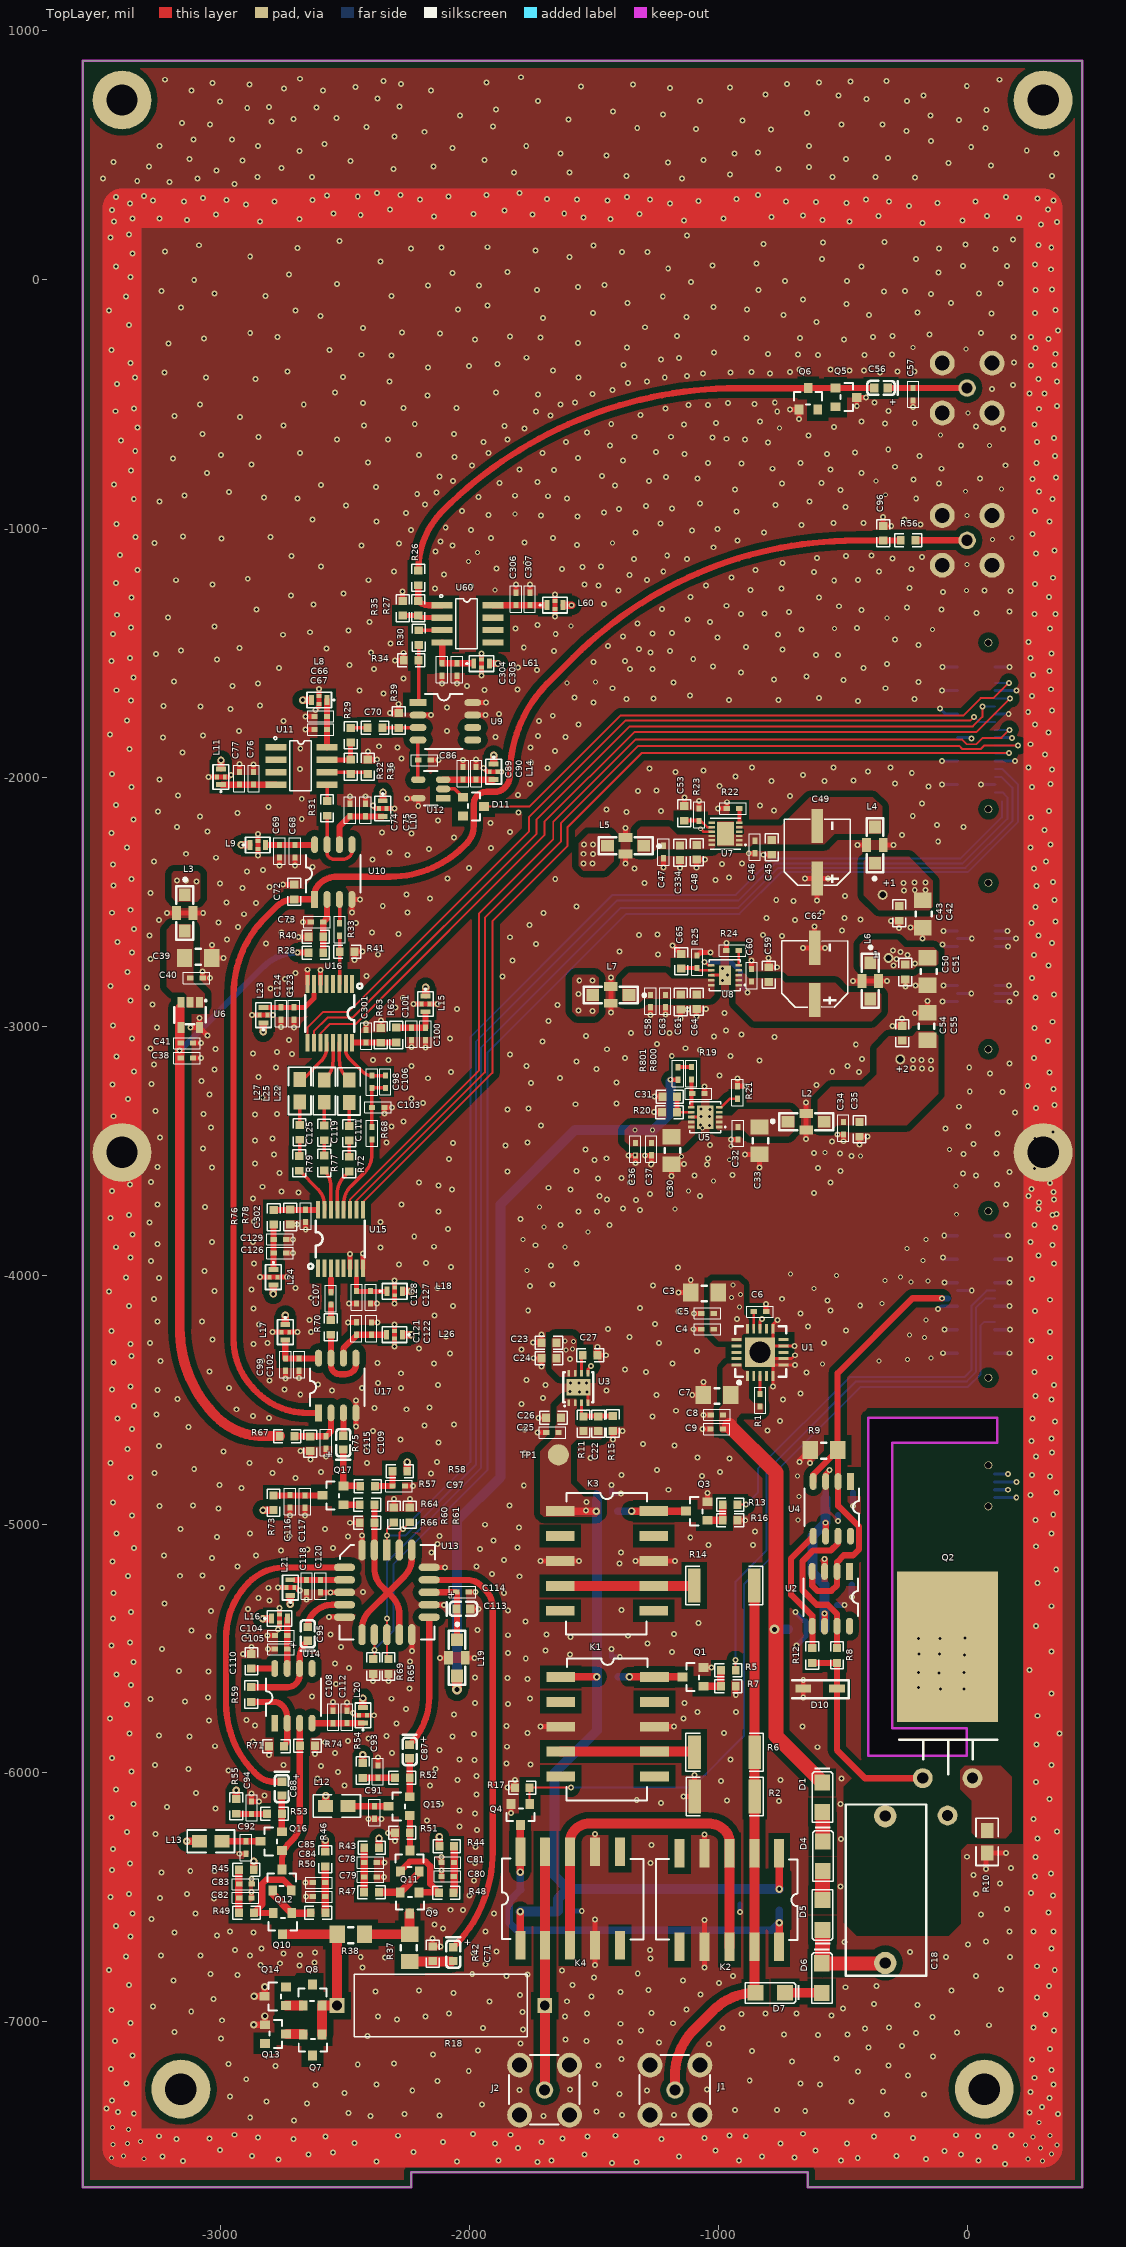
[diagram p0: TopLayer view]
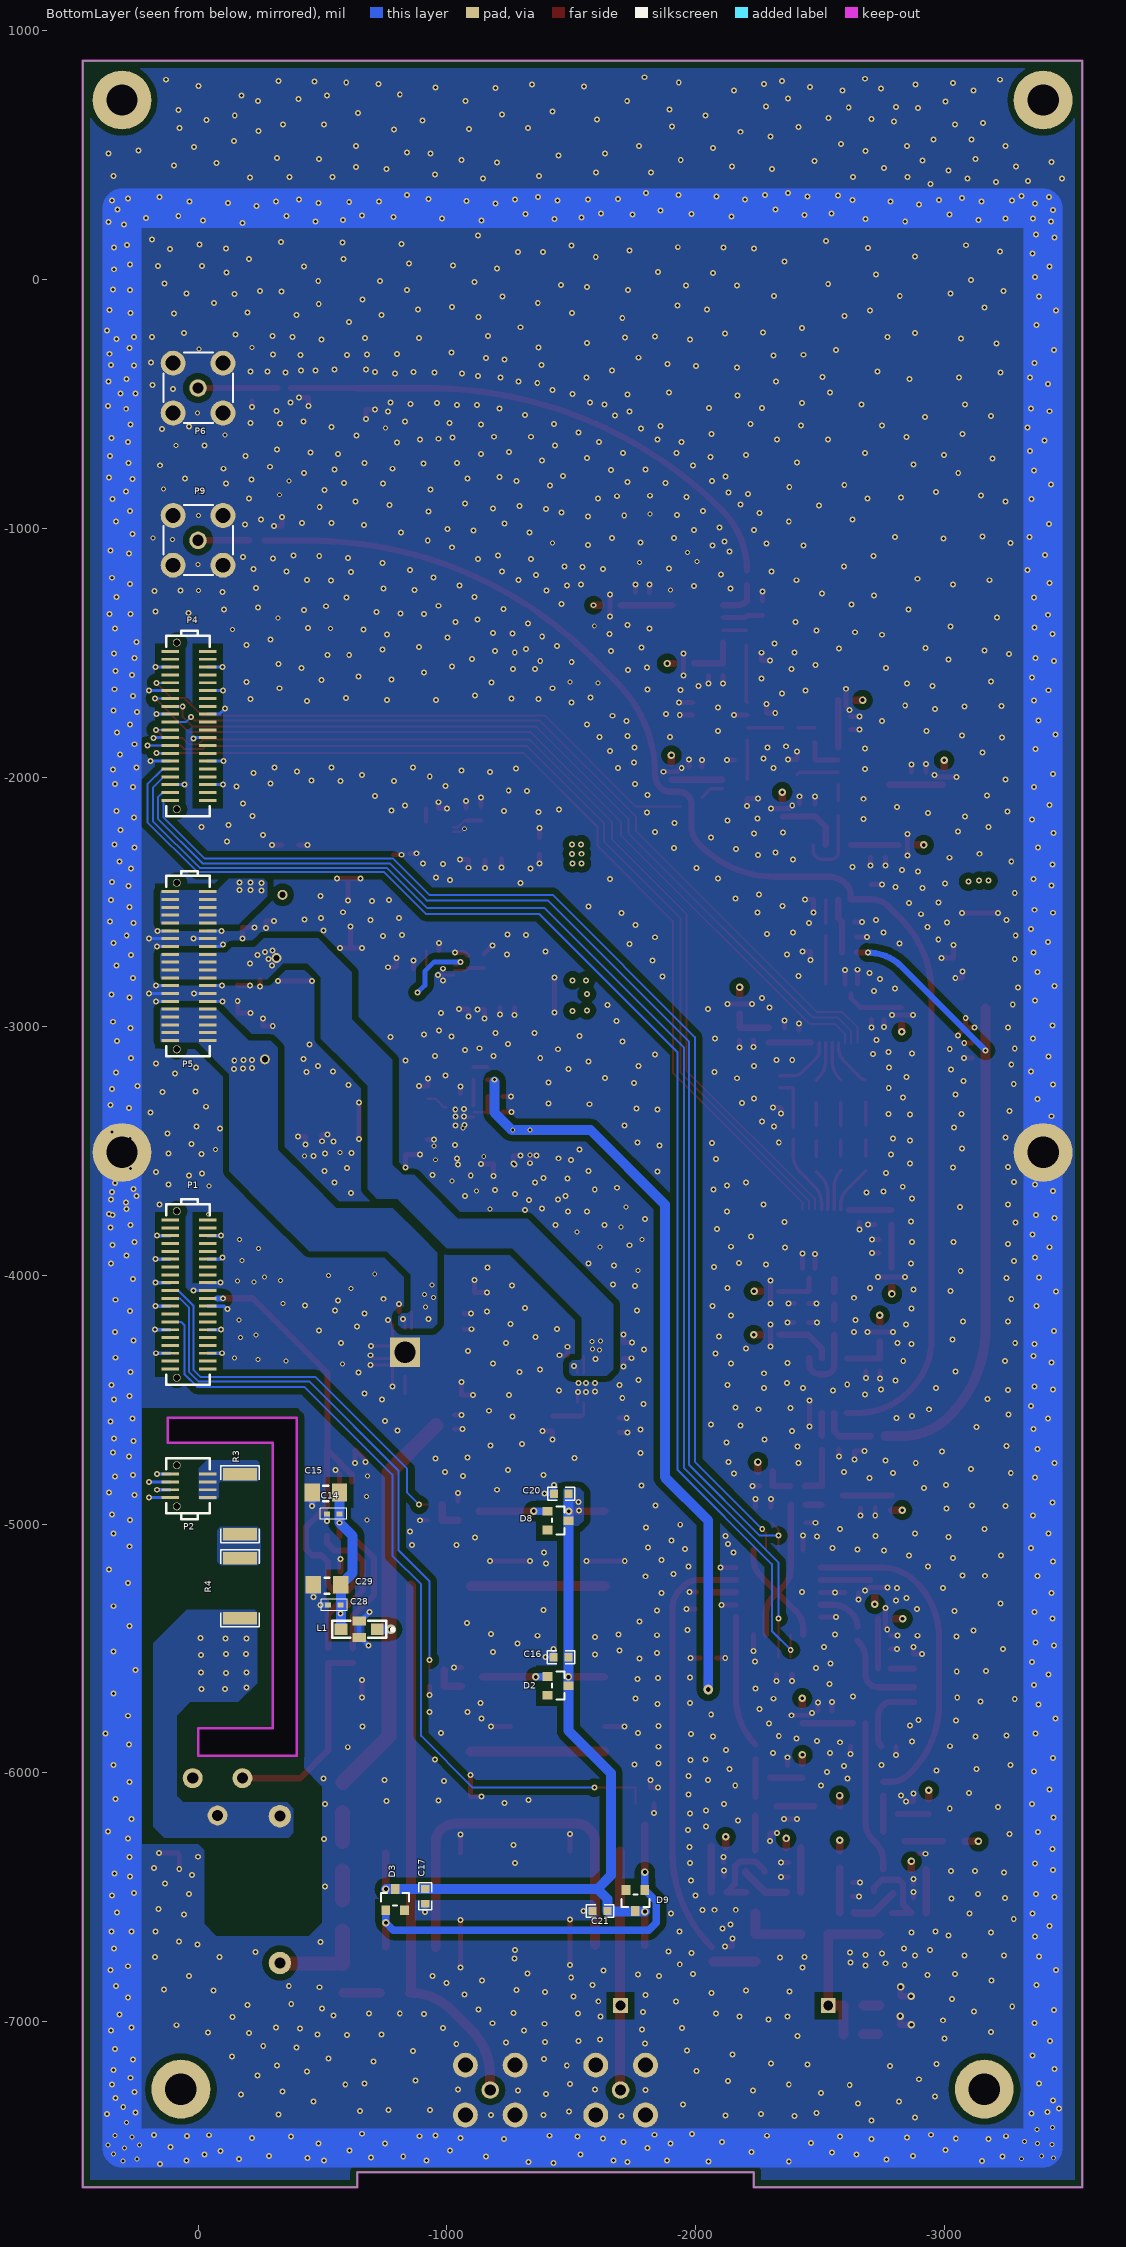
[diagram p1: BottomLayer view, seen from below]
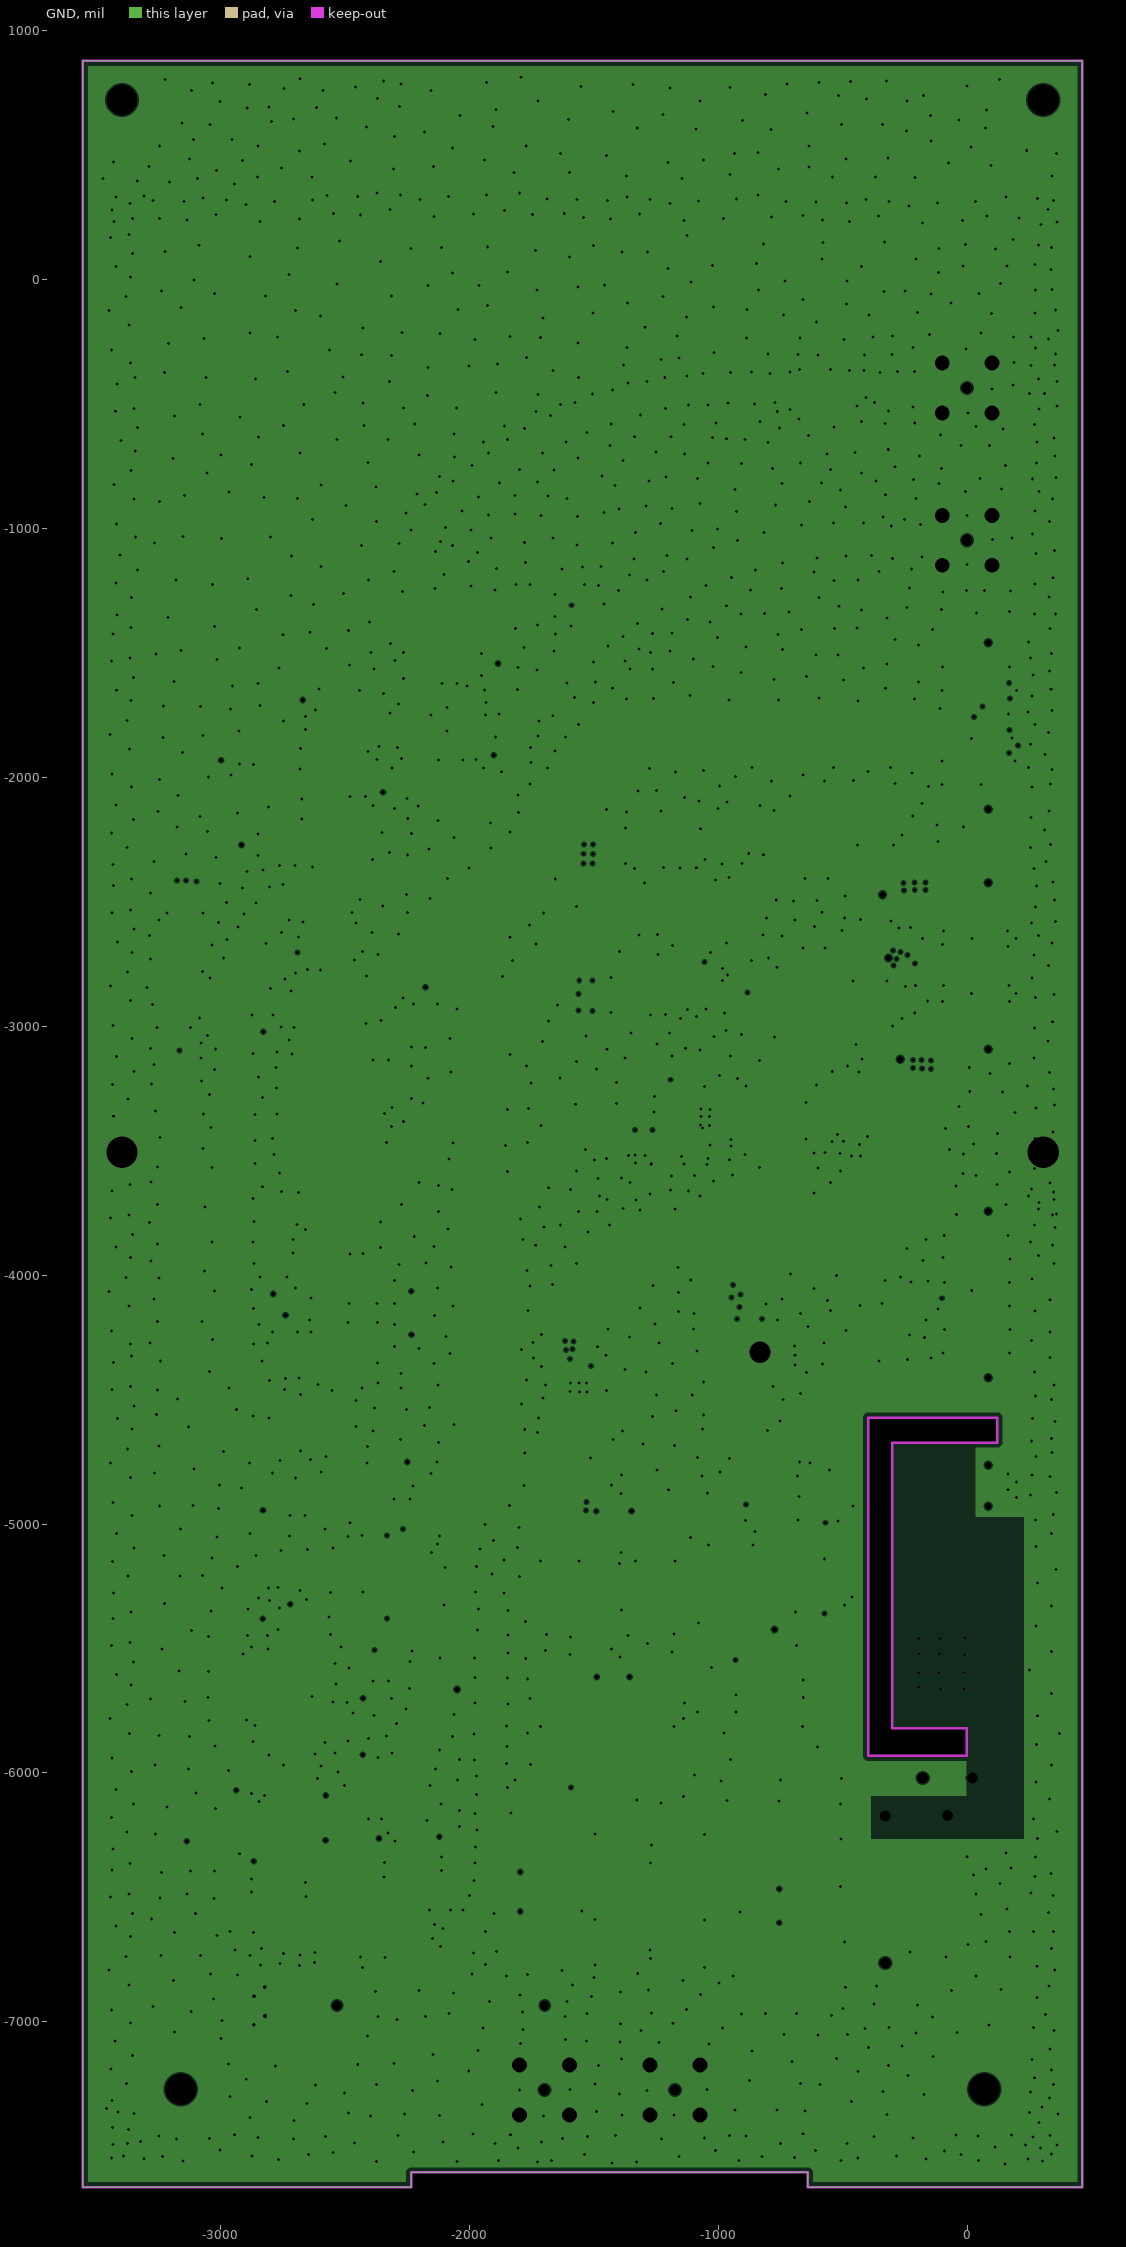
[diagram p2: GND, clearances drawn from the general rule]
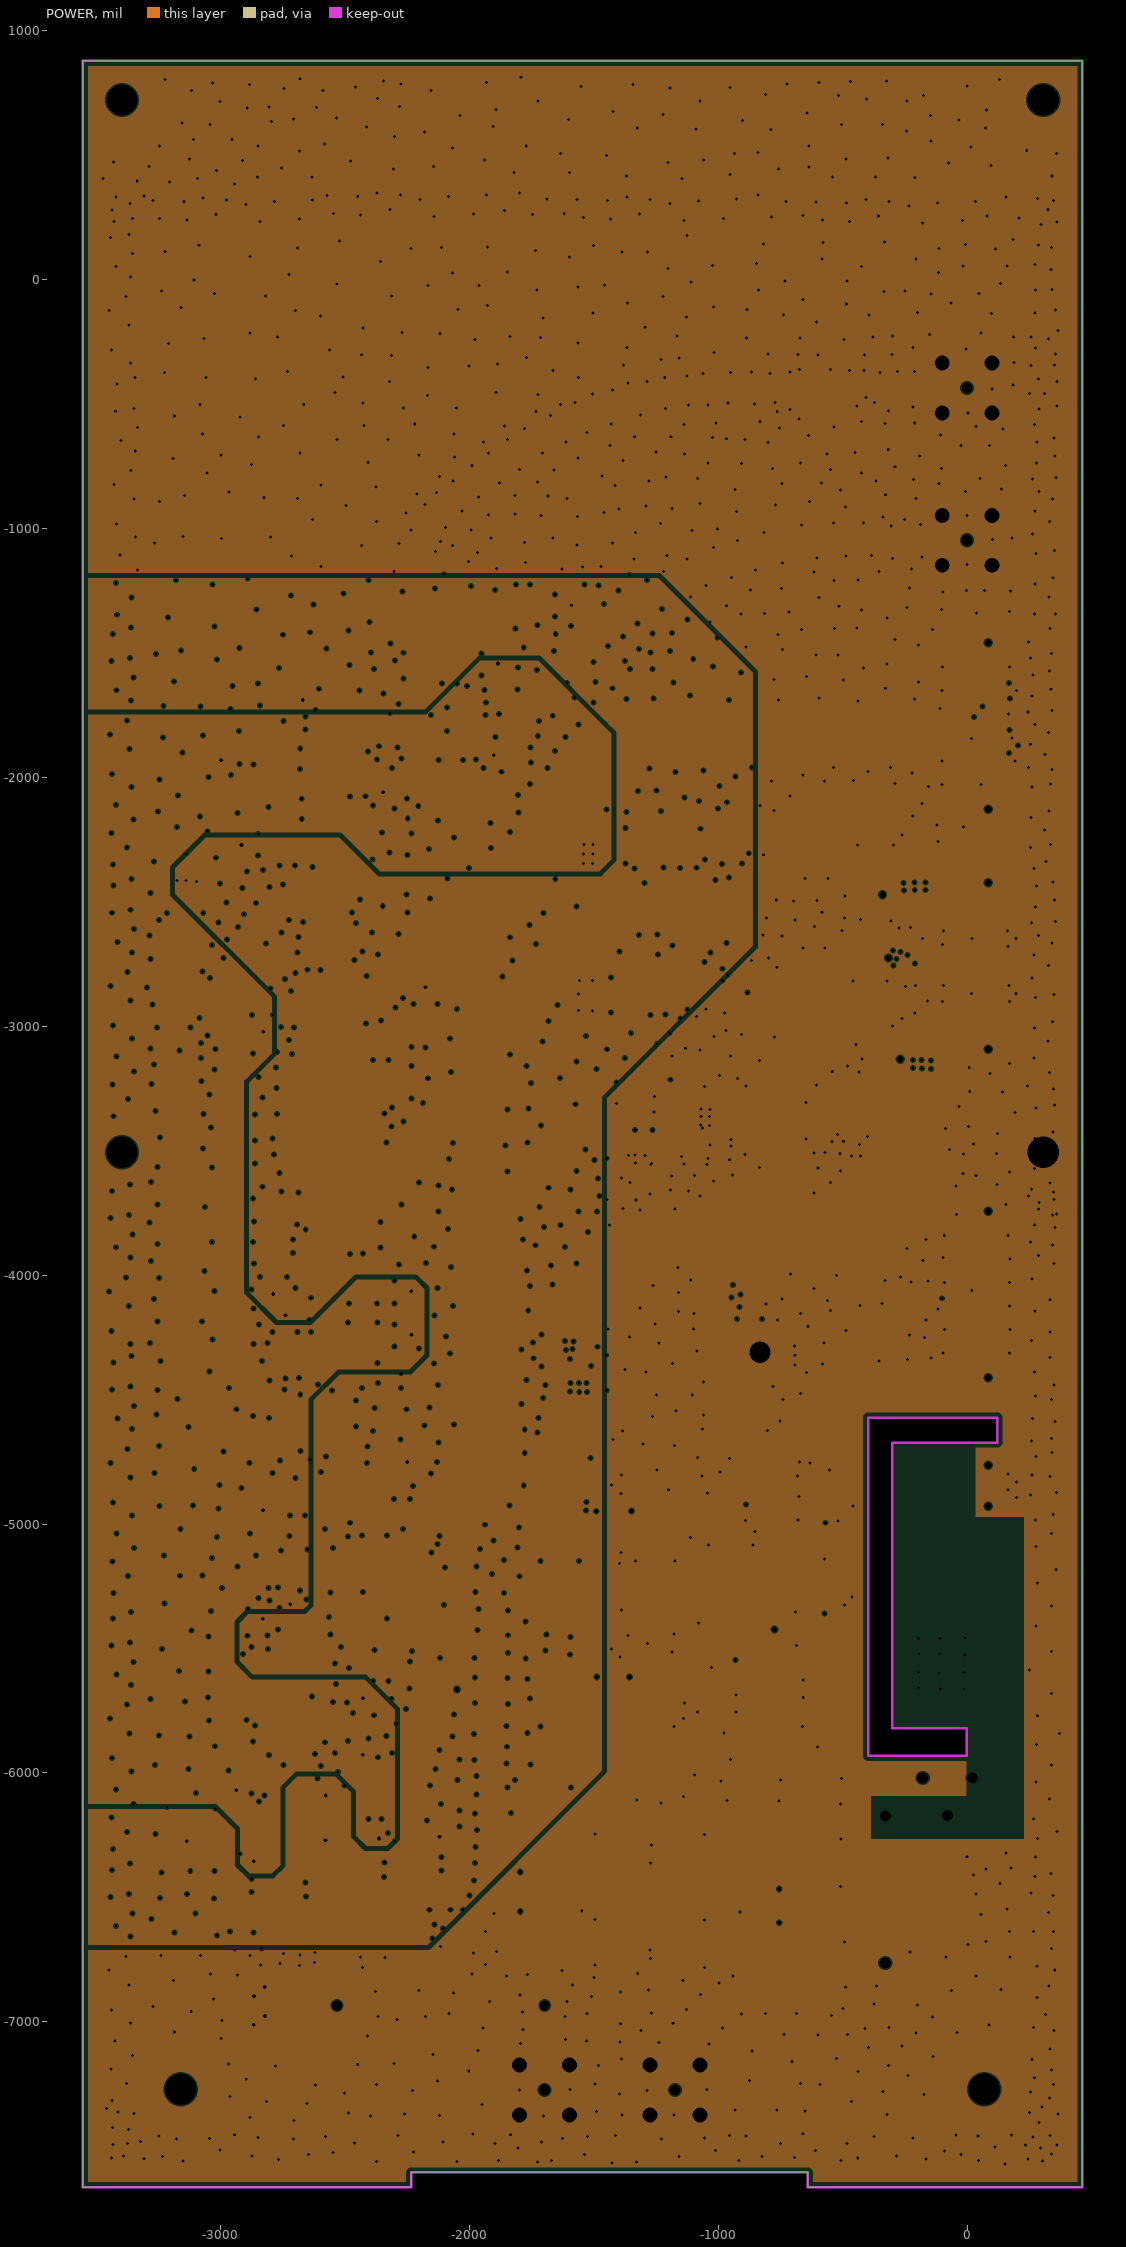
[diagram p3: POWER, clearances drawn from the general rule]
# Altium PCB MISC109358.PcbDoc (part 1 of 7)
Units mil, origin at the board's own origin, x right, y up, seen from the top; angles counter-clockwise.
Board outline 4015.75 x 8543.31 mil, 4 copper layers (TopLayer, GND, POWER, BottomLayer), stack 33.234 mil thick; 299 components, 170 nets, 998 pads, 2318 vias.

## Layer stack, top to bottom
TopLayer: signal copper 1.4
Dielectric: core 12.6, FR-4, Dk 4.8
GND: plane copper 1.417, net GND
Dielectric: prepreg 5, Dk 4.2
POWER: plane copper 1.417, net (Multiple Nets)
Dielectric: core 10, Dk 4.2
BottomLayer: signal copper 1.4

## Board outline
-3553,-7664 -3553,879.31 462.75,879.31 462.75,-7664 -640.3,-7664 -640.3,-7604.94 -2233.7,-7604.94 -2233.7,-7664
cut-out: -397.52,-5931.52 -397.52,-4572.52 121.48,-4572.52 121.48,-4672.52 -301.14,-4672.52 -301.14,-5819.52 -1.52,-5819.52 -1.52,-5931.52

## Design rules (kind name [scope] priority, off if disabled: settings)
Clearance Clearance_3 [ispad vs ispad] p1: gap=6
Clearance Clearance_2 [inpolygon] p2: gap=6
Clearance Clearance_1 [(IsKeepOut)] p3 off: gap=6
Clearance [All] p4: gap=6
ComponentClearance [All] p1 off: gap=10 collisioncheckmode=3 verticalgap=10 showdistances=FALSE
DiffPairsRouting [All] p1: maxlimit=6 minlimit=6 mostfreqgap=6 maxuncoupledlength=500
FabricationTestPointUsage TestPointUsage [All] p1: valid=0 allowmultiple=FALSE
FabricationTestpoint Testpoint [All] p1: side=3 testpointundercomponent=TRUE minsize=40 maxsize=100 preferedsize=60 minholesize=20 maxholesize=40 preferedholesize=32 testpointgrid=1 allowsidetop=TRUE allowsidebottom=TRUE usegrid=TRUE gridtolerance=0.01
HoleSize [All] p1 off: absolutevalues=TRUE maxlimit=500 minlimit=1 maxpercent=80.000 minpercent=20.000
HoleToHoleClearance [All] p1: gap=0 allowstackedmicrovias=TRUE
MinimumSolderMaskSliver [All] p1: minsoldermaskwidth=0
PlaneClearance [All] p1: clearance=6
PlaneConnect [All] p1: planeconnectstyle=Direct reliefexpansion=20 reliefentries=4 reliefconductorwidth=10 reliefairgap=10
PolygonConnect [All] p1: connectstyle=Direct reliefconductorwidth=10 reliefentries=4 polygonreliefangle="90 Angle"
RoutingVias [All] p1: holewidth=12 width=20 viastyle="Through Hole" minholewidth=12 minwidth=20 maxholewidth=20 maxwidth=40
SilkToSilkClearance [All] p1: silktosilkclearance=0
SilkscreenOverComponentPads [IsPad] p1: minsilkscreentomaskgap=0
SolderMaskExpansion [All] p1: expansion=4
Width [All] p1: maxlimit=200 minlimit=8 preferedwidth=10 minimp=50.000000 maximp=50.000000 favimp=50.000000
17 further rules are at their usual default settings.

## Components (designator, comment, footprint, x,y, rotation, side; value= is the part's Value field where it differs from the comment)
1 "" DIP-1 -315.52,-2725.52 r90 top
+1 "" DIP-1 -339.52,-2471.52 r0 top
+2 "" DIP-1 -268.52,-3132.52 r0 top
C3 "47uF 25V" 1206 -1000.52,-4069.52 r270 top
C4 "0.1uF" 0402 -1018,-4217 r180 top
C5 "1uF 25V" 0402 -1018.52,-4153.52 r180 top
C6 "1uF 25V" 0402 -857.41,-4146.52 r0 top
C7 "47uF 25V" 1206 -949.52,-4481.52 r270 top
C8 "0.1uF" 0402 -980.52,-4561.52 r180 top
C9 "1uF 25V" 0402 -981,-4618.52 r180 top
C14 "0.1uF" 0402 -568.52,-4958.52 r0 bottom
C15 "47uF 25V" 1206 -568.52,-4872.52 r270 bottom
C16 "10uF 10V" 0603 -1428.52,-5534.52 r180 bottom
C17 "10uF 10V" 0603 -912.52,-6525.52 r90 bottom
C18 "0.1uF 5% 630V" AXIAL0.59 -328.52,-6173.52 r270 top
C20 "10uF 10V" 0603 -1429.52,-4877.52 r180 bottom
C21 "10uF 10V" 0603 -1585.52,-6554.52 r180 bottom
C22 "10nF" 0603 -1482.48,-4566.96 r270 top
C23 "22uF 16V" 0603 -1709.79,-4270.52 r0 top
C24 "0.1uF" 0603 -1650.48,-4333.52 r180 top
C25 "0.1uF" 0402 -1641.48,-4632.48 r180 top
C26 "22uF 16V" 0603 -1632.48,-4572.96 r180 top
C27 "0.1uF" 0603 -1544.52,-4321.52 r0 top
C28 "0.1uF" 0402 -572.51,-5325.11 r0 bottom
C29 "47uF 25V" 1206 -573.52,-5243.52 r270 bottom
C30 "47uF 25V" 1206 -1187.26,-3443.69 r0 top
C31 "4.7uF 25V" 0603 -1165.38,-3282.73 r180 top
C32 "0.1uF" 0402 -920.52,-3404.52 r270 top
C33 "47uF 25V" 1206 -834.52,-3404.52 r0 top
C34 "0.1uF" 0402 -497.38,-3384.09 r270 top
C35 "4.7uF 25V" 0603 -432.52,-3384.09 r270 top
C36 "0.1uF" 0402 -1333.02,-3468.52 r270 top
C37 "0.1uF" 0402 -1268.4,-3468.21 r270 top
C38 "4.7uF 10V" 0402 -3109.97,-3127.35 r180 top
C39 "47uF 25V" 1206 -3144.52,-2724.52 r90 top
C40 "0.1uF" 0402 -3071.52,-2806.52 r180 top
C41 "0.1uF" 0402 -3109.97,-3067.83 r180 top
C42 "47uF 25V" 1206 -178.49,-2493.52 r0 top
C43 "0.1uF" 0603 -273.52,-2516.52 r270 top
C45 "22uF 16V" 0603 -785.52,-2310.52 r90 top
C46 "0.1uF" 0402 -852.52,-2254.52 r270 top
C47 "0.1uF" 0402 -1219.27,-2274.52 r270 top
C48 "22uF 16V" 0603 -1086.75,-2330.28 r90 top
C49 "220UF10V (D6.3*7.7mm)" CAP-SMD_BD6.3-L6.6-W6.6-FD -602.52,-2405.52 r90 top
C50 "0.1uF" 0603 -248.52,-2811.52 r90 top
C51 "47uF 25V" 1206 -158.52,-2724.09 r0 top
C53 "22uF 16V" 0603 -1136.52,-2173.83 r90 top
C54 "0.1uF" 0603 -261.52,-3057.52 r90 top
C55 "47uF 25V" 1206 -159.52,-3055.52 r180 top
C56 "2.2UF 10V" 0603钽电容 -318.52,-434.89 r180 top
C57 "10pF" 0402 -217,-485.37 r90 top
C58 "0.1uF" 0402 -1271.75,-2873.52 r270 top
C59 "22uF 16V" 0603 -797.52,-2762.52 r270 top
C60 "0.1uF" 0402 -865.75,-2820 r90 top
C61 "22uF 16V" 0603 -1151.23,-2932 r90 top
C62 "220UF10V (D6.3*7.7mm)" CAP-SMD_BD6.3-L6.6-W6.6-FD -612.52,-2894.52 r90 top
C63 "10nF" 0402 -1212.75,-2873.52 r270 top
C64 "22uF 16V" 0603 -1087.23,-2931 r90 top
C65 "22uF 16V" 0603 -1149.52,-2708.52 r270 top
C66 "4.7uF 10V" 0402 -2622,-1754.08 r0 top
C67 "0.1uF" 0402 -2572,-1808 r180 top
C68 "4.7uF 10V" 0402 -2701.01,-2321.09 r90 top
C69 "0.1uF" 0402 -2762.35,-2271.09 r270 top
C70 "10nF" 0603 -2349.52,-1800.52 r180 top
C71 "1UF 20V" 0603钽电容 -2064.52,-6700.52 r270 top
C72 "NC" 0603 -2704.52,-2489.52 r90 top
C73 "0.1uF" 0402 -2587.52,-2581.52 r180 top
C74 "0.1uF" 0402 -2479.89,-2155.95 r90 top
C75 "4.7uF 10V" 0402 -2416.55,-2105.95 r270 top
C76 "0.1uF" 0402 -2866.52,-2028.52 r90 top
C77 "4.7uF 10V" 0402 -2924.52,-1978.52 r270 top
C78 "4.7uF 10V" 0402 -2372.52,-6360.52 r180 top
C79 "0.1uF" 0402 -2372.52,-6417.52 r180 top
C80 "0.1uF" 0402 -2062.52,-6415.52 r180 top
C81 "4.7uF 10V" 0402 -2112.04,-6359 r0 top
C82 "4.7uF 10V" 0402 -2875.04,-6502.04 r180 top
C83 "0.1uF" 0402 -2924.52,-6446.52 r0 top
C84 "0.1uF" 0402 -2629,-6496.48 r0 top
C85 "4.7uF 10V" 0402 -2629,-6440 r0 top
C86 "10pF" 0402 -2205.52,-1930.52 r0 top
C87 "1UF 20V" 0603钽电容 -2240.02,-5885.88 r270 top
C88 "1UF 20V" 0603钽电容 -2753.52,-6035.52 r270 top
C89 "4.7uF 10V" 0402 -2025.04,-1958.46 r270 top
C90 "0.1uF" 0402 -1973.04,-2008.46 r90 top
C91 "0.1uF" 0402 -2380.52,-6134 r270 top
C92 "0.1uF" 0402 -2897,-6274.48 r270 top
C93 "0.1uF" 0402 -2368.04,-5969.48 r270 top
C94 "0.1uF" 0402 -2874.52,-6114.48 r270 top
C95 "10uF 10V" 0603钽电容 -2649.52,-5468.52 r90 top
C96 "NC" 0603 -337.61,-1048.18 r90 top
C97 "0.1uF" 0402 -2258.52,-4847.52 r180 top
C98 "2.2nF 1%" 0402 -2390.96,-3198 r270 top
C99 "0.1uF" 0402 -2739.52,-4384.04 r90 top
C100 "4.7uF 10V" 0402 -2176.52,-3055.52 r90 top
C101 "0.1uF" 0402 -2232.02,-3005.52 r270 top
C102 "4.7uF 10V" 0402 -2684.04,-4384.04 r90 top
C103 "2.2nF 1%" 0402 -2341.52,-3325.52 r180 top
C104 "4.7uF 10V" 0402 -2781.52,-5447.52 r0 top
C105 "0.1uF" 0402 -2782,-5502 r0 top
C106 "1.2nF 1%" 0402 -2337,-3197.52 r270 top
C107 "0.1uF" 0402 -2556,-4068 r270 top
C108 "0.1uF" 0402 -2547.04,-5750 r270 top
C109 "2.2UF 10V" 0603钽电容 -2506.52,-4700.52 r90 top
C110 "0.1uF" 0603 -2875.52,-5521.17 r270 top
C111 "270pF 1%" 0603 -2483.48,-3400 r270 top
C112 "4.7uF 10V" 0402 -2491.52,-5749.52 r270 top
C113 "1UF 20V" 0603钽电容 -2051.52,-5340.52 r0 top
C114 "0.1uF" 0402 -2002.52,-5273.52 r180 top
C115 "0.1uF" 0402 -2575.52,-4647.21 r270 top
C116 "0.1uF" 0402 -2721.04,-4933.52 r90 top
C117 "4.7uF 10V" 0402 -2661.04,-4934.52 r90 top
C118 "0.1uF" 0402 -2653.52,-5274.12 r90 top
C119 "100pF 1%" 0603 -2582.52,-3398.52 r270 top
C120 "4.7uF 10V" 0402 -2598.77,-5274.02 r90 top
C121 "0.1uF" 0402 -2453.52,-4189 r270 top
C122 "4.7uF 10V" 0402 -2394.08,-4189.52 r270 top
C123 "4.7uF 10V" 0402 -2705.04,-2973.04 r90 top
C124 "0.1uF" 0402 -2756.04,-2923.04 r270 top
C125 "56pF 1%" 0603 -2682.48,-3396.31 r270 top
C126 "0.1uF" 0402 -2736,-3911.52 r180 top
C127 "4.7uF 10V" 0402 -2396.52,-4113.52 r90 top
C128 "0.1uF" 0402 -2453.52,-4113.52 r90 top
C129 "4.7uF 10V" 0402 -2736,-3856.04 r180 top
C301 "0.1uF" 0402 -2414.52,-3064.52 r90 top
C302 "0.1uF" 0402 -2657.52,-3786.52 r90 top
C304 "0.1uF" 0402 -2109.23,-1540.99 r270 top
C305 "4.7uF 10V" 0402 -2050.52,-1591.04 r90 top
C306 "0.1uF" 0402 -1813.52,-1307.48 r90 top
C307 "4.7uF 10V" 0402 -1757.31,-1257.48 r270 top
C334 "22uF 16V" 0603 -1153.75,-2332.28 r90 top
D1 "ES1D SMA" 1606D -546.52,-6270.52 r270 top
D2 "MMBD914LT1G" SOT23 -1403.52,-5612.39 r270 bottom
D3 "MMBD914LT1G" SOT23 -754.52,-6551.52 r180 bottom
D4 "ES1D SMA" 1606D -544.52,-6507.52 r270 top
D5 "3SMAJ5929B" 1606D -616.52,-6397.52 r90 top
D6 "DFLU1400-7" 1606D -548.25,-6997.52 r270 top
D7 "ES1D SMA" 1606D -964.52,-6918.52 r180 top
D8 "MMBD914LT1G" SOT23 -1403.52,-4948.52 r270 bottom
D9 "MMBD914LT1G" SOT23 -1794.52,-6469.52 r0 bottom
D10 "MMSZ5248B" 1206D -523.52,-5661.52 r180 top
D11 "MMBZ5231B" SOT23 -2025.52,-2079.52 r270 top
J1 "RF connector right-angle socket" DIP-P -1274,-7374 r90 top locked
J2 "RF connector right-angle socket" DIP-P -1798,-7374 r90 top locked
K1 "TQ2SS-5V(ATQ209SS)SMD10" K -1632.52,-5614.52 r0 top
K2 "TQ2SS-5V(ATQ209SS)SMD10" K -755.52,-6322 r270 top
K3 "TQ2SS-5V(ATQ209SS)SMD10" K -1635.52,-4948.52 r0 top
K4 "TQ2SS-5V(ATQ209SS)SMD10" K -1795.08,-6692.52 r90 top
L1 "YFF31HC2A105MT000N" FILTER-SMD_4P-L3.2-W1.6-L_YFF31HC -720.52,-5422.52 r0 bottom
L2 "YFF31HC2A105MT000N" FILTER-SMD_4P-L3.2-W1.6-L_YFF31HC -719.38,-3383.09 r0 top
L3 "YFF31HC2A105MT000N" FILTER-SMD_4P-L3.2-W1.6-L_YFF31HC -3143.52,-2471.52 r270 top
L4 "YFF31HC2A105MT000N" FILTER-SMD_4P-L3.2-W1.6-L_YFF31HC -370.52,-2344.52 r90 top
L5 "YFF31HC2A105MT000N" FILTER-SMD_4P-L3.2-W1.6-L_YFF31HC -1299.52,-2274.52 r180 top
L6 "YFF31HC2A105MT000N" FILTER-SMD_4P-L3.2-W1.6-L_YFF31HC -389.52,-2744.52 r270 top
L7 "YFF31HC2A105MT000N" FILTER-SMD_4P-L3.2-W1.6-L_YFF31HC -1359,-2873.52 r180 top
L8 "NFM18PC104R1C3D" FILTER-SMD_3P-L1.6-W0.8-L_NFM18CC223R1C3D -2572,-1688.52 r180 top
L9 "NFM18PC104R1C3D" FILTER-SMD_3P-L1.6-W0.8-L_NFM18CC223R1C3D -2881.52,-2271.52 r0 top
L10 "NFM18PC104R1C3D" FILTER-SMD_3P-L1.6-W0.8-L_NFM18CC223R1C3D -2348.08,-2093.52 r270 top
L11 "NFM18PC104R1C3D" FILTER-SMD_3P-L1.6-W0.8-L_NFM18CC223R1C3D -2998.52,-2029 r90 top
L12 "0.39UH 10%" 0805 -2577.52,-6132.52 r0 top
L13 "0.39UH 10%" 0805 -3083.52,-6274.52 r0 top
L14 "NFM18PC104R1C3D" FILTER-SMD_3P-L1.6-W0.8-L_NFM18CC223R1C3D -1902.52,-1945.52 r270 top
L15 "NFM18PC104R1C3D" FILTER-SMD_3P-L1.6-W0.8-L_NFM18CC223R1C3D -2176.52,-2878.52 r270 top
L16 "NFM18PC104R1C3D" FILTER-SMD_3P-L1.6-W0.8-L_NFM18CC223R1C3D -2794.52,-5379.52 r0 top
L17 "NFM18PC104R1C3D" FILTER-SMD_3P-L1.6-W0.8-L_NFM18CC223R1C3D -2739.52,-4197.52 r270 top
L18 "NFM18PC104R1C3D" FILTER-SMD_3P-L1.6-W0.8-L_NFM18CC223R1C3D -2331.52,-4064.52 r0 top
L19 "YFF31HC2A105MT000N" FILTER-SMD_4P-L3.2-W1.6-L_YFF31HC -2050.04,-5464.52 r270 top
L20 "NFM18PC104R1C3D" FILTER-SMD_3P-L1.6-W0.8-L_NFM18CC223R1C3D -2427.52,-5799.52 r90 top
L21 "NFM18PC104R1C3D" FILTER-SMD_3P-L1.6-W0.8-L_NFM18CC223R1C3D -2719.52,-5286.52 r90 top
L22 "18UH 5%" 0805 -2483.48,-3306 r90 top
L23 "NFM18PC104R1C3D" FILTER-SMD_3P-L1.6-W0.8-L_NFM18CC223R1C3D -2827.52,-2986.52 r90 top
L24 "NFM18PC104R1C3D" FILTER-SMD_3P-L1.6-W0.8-L_NFM18CC223R1C3D -2787.52,-3976.52 r270 top
L25 "10UH 5%" 0805 -2582.48,-3305 r90 top
L26 "NFM18PC104R1C3D" FILTER-SMD_3P-L1.6-W0.8-L_NFM18CC223R1C3D -2269.52,-4239 r180 top
L27 "3.9UH 5%" 0805 -2681.48,-3304 r90 top
L60 "NFM18PC104R1C3D" FILTER-SMD_3P-L1.6-W0.8-L_NFM18CC223R1C3D -1687.52,-1307.48 r0 top
L61 "NFM18PC104R1C3D" FILTER-SMD_3P-L1.6-W0.8-L_NFM18CC223R1C3D -1982.52,-1542.52 r0 top
P1 "Header 20X2" N0.8mm/40Pin-Plug 111.04,-3778 r270 bottom locked
P2 "Header 4X2" N0.8mm/8Pin-SOCKET 111.04,-4893.41 r270 bottom locked
P4 "Header 20X2" N0.8mm/40Pin-Plug 111.04,-1493.52 r270 bottom locked
P5 "Header 20X2" N0.8mm/40Pin-Plug 111.04,-2458.63 r270 bottom locked
P6 "RF connector straight jack" DIP-P 100,-335.37 r180 bottom locked
P9 "RF connector straight jack" DIP-P 100,-947.18 r180 bottom locked
Q1 "PMBT3904" SOT23 -1058.52,-5651.52 r90 top
Q2 "STP10NK80Z" TO220 21.48,-6020.52 r90 top
Q3 "PMBT3904" SOT23 -1044,-4985 r90 top
Q4 "2N7002-7-F" SOT23 -1757.52,-6124.52 r180 top
Q5 "MMBD914LT1G" SOT23 -528.52,-435.37 r270 top
Q6 "MMBD914LT1G" SOT23 -675.52,-520.89 r0 top
Q7 "MMBD7000LT1" SOT23 -2592.58,-7050.52 r180 top
Q8 "MMBD7000LT1" SOT23 -2667.58,-6934.52 r0 top
Q9 "MMBD7000LT1" SOT23 -2202.52,-6479.52 r180 top
Q10 "MMBD7000LT1" SOT23 -2713.52,-6563 r180 top
Q11 "MMBD7000LT1" SOT23 -2276.52,-6396.52 r0 top
Q12 "MMBD7000LT1" SOT23 -2790.52,-6473 r0 top
Q13 "MMBZ5257BLT1G" SOT23 -2821.58,-7011.52 r270 top
Q14 "MMBZ5257BLT1G" SOT23 -2737.58,-6934.52 r90 top
Q15 "PMBT3904" SOT23 -2239.52,-6171 r90 top
Q16 "PMBT3904" SOT23 -2753.52,-6311.48 r90 top
Q17 "BFT92" SOT23 -2505.48,-4922 r90 top
R1 "0R" 0402 -831.82,-4527.52 r90 top
R2 "470R 5% 1W" 2512 -853.52,-6094.52 r180 top
R3 "1K 1W" 2512 -168.52,-5041.52 r90 bottom
R4 "1K 1W" 2512 -168.52,-5137.52 r270 bottom
R5 "2.21K 1%" 0603 -989,-5587.52 r0 top
R6 "220R 5% 1W" 2512 -1095.52,-5916.52 r0 top
R7 "10K 1%" 0603 -989,-5651.04 r0 top
R8 "1.5R" 0603 -522.93,-5557.24 r90 top
R9 "1.15K 1%" 1206 -520.52,-4701.52 r270 top
R10 "0.5R 1%" 0805 80.48,-6321.52 r90 top
R11 "52.5K 1%" 0603 -1541.48,-4566.96 r270 top
R12 "1.5R" 0603 -621.51,-5557.76 r90 top
R13 "2.21K 1%" 0603 -982.14,-4921.52 r0 top
R14 "82R 5% 3W" 2512 -1096.52,-5246.52 r0 top
R15 "10K 1%" 0603 -1423.48,-4565.96 r270 top
R16 "10K 1%" 0603 -982,-4984.52 r0 top
R17 "10K 1%" 0603 -1817.04,-6058.52 r0 top
R18 "51R 5W" 5W -1697.52,-6934.52 r180 top
R19 "13.3K  1%" 0402 -1104.9,-3270.21 r0 top
R20 "121K" 0603 -1166.38,-3344.73 r180 top
R21 "0R" 0402 -923.52,-3290.52 r90 top
R22 "0R" 0402 -915.52,-2125.52 r180 top
R23 "49.9K 1%" 0402 -1077,-2174.59 r90 top
R24 "0R" 0402 -917.75,-2695.52 r180 top
R25 "49.9K 1%" 0402 -1084.58,-2765.83 r90 top
R26 "47R 1%" 0603 -2205.52,-1227.52 r90 top
R27 "681R 1%" 0603 -2205.52,-1290.52 r270 top
R28 "22.1K 1%" 0603 -2646.52,-2703.52 r0 top
R29 "10R 1%" 0603 -2477,-1800.52 r270 top
R30 "100R 1%" 0603 -2203.52,-1408.52 r270 top
R31 "100R 1%" 0603 -2572,-2094.52 r270 top
R32 "681R 1%" 0603 -2477,-1927.52 r270 top
R33 "0R" 0402 -2521.52,-2635.52 r90 top
R34 "1K 1%" 0603 -2204.52,-1529.52 r180 top
R35 "681R 1%" 0603 -2268.52,-1349.83 r90 top
R36 "100R 1%" 0603 -2407.52,-1986.52 r90 top
R37 "90.9R 1%" 1206 -2239.52,-6757.52 r180 top
R38 "909R 1%" 1206 -2421.52,-6648 r270 top
R39 "1.21K 1%" 0603 -2284.52,-1800.52 r90 top
R40 "5.62K 1%" 0603 -2646.52,-2640.52 r0 top
R41 "10K 1%" 0603 -2461.52,-2699.52 r180 top
R42 "10R 1%" 0603 -2147.52,-6696.52 r270 top
R43 "1.21K 1%" 0603 -2422.52,-6299.52 r0 top
R44 "1.21K 1%" 0603 -2120.52,-6293.52 r0 top
R45 "1.21K 1%" 0603 -2866.52,-6389.52 r180 top
R46 "1.21K 1%" 0603 -2578.52,-6316.52 r270 top
R47 "3.32K 1%" 0603 -2363.52,-6478.52 r180 top
R48 "3.32K 1%" 0603 -2063.52,-6480.52 r180 top
R49 "3.32K 1%" 0603 -2925.41,-6562 r0 top
R50 "3.32K 1%" 0603 -2637.52,-6562 r0 top
R51 "4.75K 1%" 0603 -2239.52,-6241 r180 top
R52 "1K 1%" 0603 -2239.52,-6018.52 r180 top
R53 "1K 1%" 0603 -2812.52,-6164.48 r0 top
R54 "49.9R 1%" 0603 -2428.52,-6019.48 r90 top
R55 "49.9R 1%" 0603 -2936.52,-6104.48 r270 top
R56 "100R 1%" 0603 -266.61,-1047.18 r0 top
R57 "301R 1%" 0603 -2438.52,-4847.52 r0 top
R58 "20R 1%" 0603 -2249.52,-4787.52 r180 top
R59 "1K 1%" 0603 -2876.52,-5714.52 r90 top
R60 "20K 1%" 0603 -2302.99,-4933.52 r270 top
R61 "20K 1%" 0603 -2238.99,-4992.52 r90 top
R62 "1K 1%" 0603 -2293.52,-3064.52 r90 top
R63 "1.21K 1%" 0603 -2355.52,-3006.52 r270 top
R64 "100R 1%" 0603 -2440.52,-4921.52 r0 top
R65 "20K 1%" 0603 -2325,-5542.23 r270 top
R66 "1K 1%" 0603 -2440.52,-4994.52 r0 top
R67 "22.1K 1%" 0603 -2702.52,-4646.52 r180 top
R68 "0R" 0402 -2392,-3454.52 r90 top
R69 "20K 1%" 0603 -2387,-5601.54 r90 top
R70 "10R 1%" 0603 -2557,-4239 r90 top
R71 "118R 1%" 0603 -2804.52,-5892.52 r0 top
R72 "0R" 0603 -2483.48,-3583.31 r90 top
R73 "20R 1%" 0603 -2787,-4884.5 r270 top
R74 "4.75K 1%" 0603 -2620.77,-5890.52 r180 top
R75 "5.62K 1%" 0603 -2638.52,-4706.52 r90 top
R76 "1K 1%" 0603 -2786.52,-3737.52 r270 top
R77 "49.9R 1%" 0603 -2583.52,-3519.52 r270 top
R78 "1.21K 1%" 0603 -2720.52,-3736.52 r270 top
R79 "10R 1%" 0603 -2683.48,-3521 r270 top
R800 "523K 1%" 0402 -1107.48,-3163.76 r270 top
R801 "4.7K 1%" 0402 -1162.48,-3214.52 r90 top
TP1 "" TP1 -1642.52,-4721.52 r0 top
U1 "TPS7A4701RGWR" QFN-20 -883,-4404 r90 top
U2 "TC4426COA(microchip)" SO8 -472.51,-5190.24 r270 top
U3 "TPL910A" DFN-8_L3.0-W3.0-P0.65-BL-EP2.3 -1600.48,-4511.96 r0 top
U4 "TC4426COA(microchip)" SO8 -468.51,-4828.65 r270 top
U5 "GM12051ACPZ-R7" TDFN-10_L3.0-W3.0-P0.50-BL-EP -1019,-3371.69 r90 top
U6 "#NAME?" TSOT-23-5_L2.9-W1.6-P0.95-LS2.8-BR -3081.97,-2888.83 r90 top
U7 "LT3094EDD#PBF" WDFN-12_L3.0-W3.0-P0.45-BL-EP -1065.75,-2281.28 r90 top
U8 "LT3045EDD#PBF" DFN-10_L3.0-W3.0-P0.50-BL-EP -917.75,-2834 r90 top
U9 "MASWSS0157TR" SO8 -2206.52,-1699.52 r0 top
U10 "AD603AR" SO8 -2622,-2490 r90 top
U11 "#NAME?" SOP8 -2777,-1879 r0 top
U12 "SN74AHC1G04DBVR" SOT25 -2105.52,-2083.52 r180 top
U13 "DG540DN PLCC20" QUAD20 -2501.52,-5174.52 r0 top
U14 "LMH6624MA(NS)" SO8 -2782,-5800 r90 top
U15 "ADG658YRQZ" TSSOP-16_L5.0-W4.4-P0.65-LS6.4-TL -2607.52,-3972.52 r90 top
U16 "ADG658YRQZ" TSSOP-16_L5.0-W4.4-P0.65-LS6.4-TL -2471,-2830 r270 top
U17 "AD603AR" SO8 -2606,-4553 r90 top
U60 "#NAME?" SOP8 -2110.31,-1308 r0 top

## Footprints (in the part's own frame and the unit in brackets; to place one, negate y for a bottom-side part, rotate by r counter-clockwise, add the part's x,y. Pads: shape width x height; smd on the part's side, far side on the other; paste and mask are expansions set on the pad)
5W [mm]
  rect 1.5x1.5 hole 1: 1(0,0) 2(21.2,0)
  silkscreen extent 1.77,-3.18 19.43,3.18
0402 [mil]
  rect 25x20 smd: 1(0,0) 2(50,0)
  silkscreen extent -28,-23 78,22
0603 [mil]
  rect 31.75x34.02 smd paste-3937.01 mask+2: 1(0,0) 2(59.31,0)
  silkscreen extent -25,-26 84,26
0603钽电容 [mm]
  rect 0.85x0.9 smd: 1(0,0) 2(1.4,0)
  silkscreen extent -1.02,-0.71 2.09,0.71
0805 [mil]
  rect 60x50 smd: 1(0,0) 2(90,0)
  silkscreen extent -50,-45 140,45
1206 [mil]
  rect 72x62 smd: 1(0,0) 2(0,-110)
  silkscreen extent -27,-65 36,-46
1206D [mil]
  rect 64x32 smd: 1(135.01,-0.13) 2(0.01,-0.13)
  silkscreen extent -47,-34 180,37
1606D [mm]
  rect 1.635x1.6 smd paste-100 mask+0.051: 1(-2.884,-0.904) 2(-5.919,-0.904)
  silkscreen extent -7.39,-1.94 -1.83,0.17
2512 [mil]
  rect 50.49x136.06 smd paste-3937.01 mask+2: 1(0,0) 2(241.44,0)
  silkscreen extent -34,-77 276,77
AXIAL0.59 [mil]
  round 90 hole 45: 1(-0.12,-0.44) 2(589.88,-0.44)
  silkscreen extent -47,-159 642,164
CAP-SMD_BD6.3-L6.6-W6.6-FD [mm]
  rect 3.5x1.2 smd: 1(0,0) 2(5.34,0)
  silkscreen extent -0.71,-3.38 6.05,3.38
DFN-8_L3.0-W3.0-P0.65-BL-EP2.3 [mm]
  rect 0.28x0.665 smd: 1(0,0) 2(0.65,0) 3(1.3,0) 4(1.95,0) 5(1.95,3.001) 6(1.3,3.001) 7(0.65,3.001) 8(0,3.001)
  rect 2.45x1.65 smd: 9(0.975,1.568)
  silkscreen extent -0.55,-0.41 2.5,3.09
DFN-10_L3.0-W3.0-P0.50-BL-EP [mm]
  rect 0.25x0.65 smd: 1(0,0) 2(0.5,0) 3(1,0) 4(1.5,0) 5(2,0) 6(2,2.823) 7(1.5,2.823) 8(1,2.823) 9(0.5,2.823) 10(0,2.823)
  rect 2x1.2 smd: 11(1,1.411)
  silkscreen extent -0.58,-0.69 2.58,2.99
DIP-1 [mil]
  round 40 hole 25: 1(0,0)
DIP-P [mil]
  round 100 hole 60: 1(0,0) 2(0,-200) 3(200,-200) 4(200,0)
  round 70 hole 45: 5(100,-100)
  silkscreen extent -39,-240 240,42
FILTER-SMD_3P-L1.6-W0.8-L_NFM18CC223R1C3D [mm]
  rect 0.5x1 smd: 1(0,0) 3(1.6,0)
  rect 0.5x0.4 smd: 2(0.8,0.4) 2(0.8,-0.4)
  silkscreen extent -0.79,-0.8 2.05,0.8
FILTER-SMD_4P-L3.2-W1.6-L_YFF31HC [mm]
  rect 1.3x1.2 smd: 1(0,0) 3(3.7,0)
  rect 1.4x0.9 smd: 2(1.85,-0.85) 4(1.85,0.85)
  silkscreen extent -1.72,-0.85 4.6,0.85
K [mil]
  rect 115x40 smd: 1(0.4,0.38) 2(0.4,-99.62) 3(0.4,-199.62) 4(0.4,-299.62) 5(0.4,-399.62) 6(376.4,-399.62) 7(376.4,-299.62) 8(376.4,-199.62) 9(376.4,-99.62) 10(376.4,0.38)
  silkscreen extent 23,-495 348,74
N0.8mm/8Pin-SOCKET [mm]
  round 0.8 hole 0.68: 0(-3.3,0.65) 0(0.9,0.65)
  rect 0.3x1.8 smd: 1(0,0) 2(0,3.8) 3(-0.8,0) 4(-0.8,3.8) 5(-1.6,0) 6(-1.6,3.8) 7(-2.4,0) 8(-2.4,3.8)
  silkscreen extent -4,-0.4 2.2,4
N0.8mm/40Pin-Plug [mm]
  round 0.8 hole 0.68: 0(-0.9,0.65) 0(16.1,0.65)
  rect 0.3x1.8 smd: 1(0,0) 2(0,3.8) 3(0.8,0) 4(0.8,3.8) 5(1.6,0) 6(1.6,3.8) 7(2.4,0) 8(2.4,3.8) 9(3.2,0) 10(3.2,3.8) 11(4,0) 12(4,3.8) 13(4.8,0) 14(4.8,3.8) 15(5.6,0) 16(5.6,3.8) 17(6.4,0) 18(6.4,3.8) 19(7.2,0) 20(7.2,3.8) 21(8,0) 22(8,3.8) 23(8.8,0) 24(8.8,3.8) 25(9.6,0) 26(9.6,3.8) 27(10.4,0) 28(10.4,3.8) 29(11.2,0) 30(11.2,3.8) 31(12,0) 32(12,3.8) 33(12.8,0) 34(12.8,3.8) 35(13.6,0) 36(13.6,3.8) 37(14.4,0) 38(14.4,3.8) 39(15.2,0) 40(15.2,3.8)
  silkscreen extent -2.1,-0.4 16.8,4
QFN-20 [mil]
  rect 40x12 smd: 1(0,0) 2(0,-25.59) 3(0,-51.18) 4(0,-76.77) 5(0,-102.36) 11(188.98,-102.36) 12(188.98,-76.77) 13(188.98,-51.18) 14(188.98,-25.59) 15(188.98,0)
  rect 12x40 smd: 6(43.31,-145.67) 7(68.9,-145.67) 8(94.49,-145.67) 9(120.08,-145.67) 10(145.67,-145.67) 16(145.67,43.31) 17(120.08,43.31) 18(94.49,43.31) 19(68.9,43.31) 20(43.31,43.31)
  rect 120x120 hole 85: 21(94.49,-51.18)
  silkscreen extent -32,-156 198,49
QUAD20 [mil]
  rect 30x85 smd: 1(170.06,70.4)
  oval 30x85 smd: 2(120.06,70.4) 3(70.06,70.4) 9(70.06,-269.6) 10(120.06,-269.6) 11(170.06,-269.6) 12(220.06,-269.6) 13(270.06,-269.6) 19(270.06,70.4) 20(220.06,70.4)
  oval 85x30 smd: 4(0.06,0.4) 5(0.06,-49.6) 6(0.06,-99.6) 7(0.06,-149.6) 8(0.06,-199.6) 14(340.06,-199.6) 15(340.06,-149.6) 16(340.06,-99.6) 17(340.06,-49.6) 18(340.06,0.4)
  silkscreen extent -20,-288 363,92
SO8 [mil]
  rect 68x28 smd: 1(0,0)
  oval 68x28 smd: 2(0,-50) 3(0,-100) 4(0,-150) 5(220,-150) 6(220,-100) 7(220,-50) 8(220,0)
  silkscreen extent 28,-185 179,35
SOP8 [mil]
  rect 85x25 smd: 1(0,0) 2(0,-50) 3(0,-100) 4(0,-150) 5(205,-150) 6(205,-100) 7(205,-50) 8(205,0)
  silkscreen extent -9,-174 142,43
SOT23 [mil]
  rect 35x40 smd: 1(0,0) 2(75,0) 3(37.5,85)
  silkscreen extent -20,19 93,69
SOT25 [mil]
  rect 58x27 smd: 1(-0.1,0.12)
  oval 58x27 smd: 2(-0.1,-37.28) 3(-0.1,-74.68) 4(99.9,-74.68) 5(99.9,0.12)
  silkscreen extent 23,-109 76,29
TDFN-10_L3.0-W3.0-P0.50-BL-EP [mm]
  rect 0.28x0.665 smd: 1(-0.821,-0.562) 2(-0.321,-0.562) 3(0.179,-0.562) 4(0.679,-0.562) 5(1.179,-0.562) 6(1.179,2.252) 7(0.679,2.252) 8(0.179,2.252) 9(-0.321,2.252) 10(-0.821,2.252)
  rect 2.4x1.7 smd: 11(0.179,0.845)
  silkscreen extent -1.4,-1.27 1.76,2.42
TO220 [mil]
  round 80 hole 45: 1(-0.18,199.97) 2(-150.18,99.97) 3(-0.18,-0.03)
  rect 605x405 smd: 4(527.82,99.97)
  silkscreen extent 16,-100 154,295
TP1 [mil]
  round 85 smd: 1(0,0)
TSOT-23-5_L2.9-W1.6-P0.95-LS2.8-BR [mm]
  rect 1.1x0.7 smd: 1(-0.357,0.065) 2(-0.357,1.015) 3(-0.357,1.967) 4(-2.945,1.967) 5(-2.945,0.067)
  silkscreen extent -2.62,-0.64 -0.13,2.62
TSSOP-16_L5.0-W4.4-P0.65-LS6.4-TL [mil]
  rect 71x16 smd: 1(0,0) 2(0,-25.6) 3(0,-51.19) 4(0,-76.78) 5(0,-102.37) 6(0,-127.96) 7(0,-153.55) 8(0,-179.14) 9(236.22,-179.14) 10(236.22,-153.55) 11(236.22,-127.96) 12(236.22,-102.37) 13(236.22,-76.78) 14(236.22,-51.19) 15(236.22,-25.6) 16(236.22,0)
  silkscreen extent -2,-188 192,40
WDFN-12_L3.0-W3.0-P0.45-BL-EP [mm]
  rect 0.252x0.665 smd: 1(0.272,-3.82) 2(0.722,-3.82) 3(1.172,-3.82) 4(1.622,-3.82) 5(2.072,-3.82) 6(2.522,-3.82) 7(2.522,-1.006) 8(2.072,-1.006) 9(1.622,-1.006) 10(1.172,-1.006) 11(0.722,-1.006) 12(0.272,-1.006)
  rect 2.4x1.7 smd: 13(1.397,-2.413)
  silkscreen extent -0.18,-4.53 2.97,-0.84